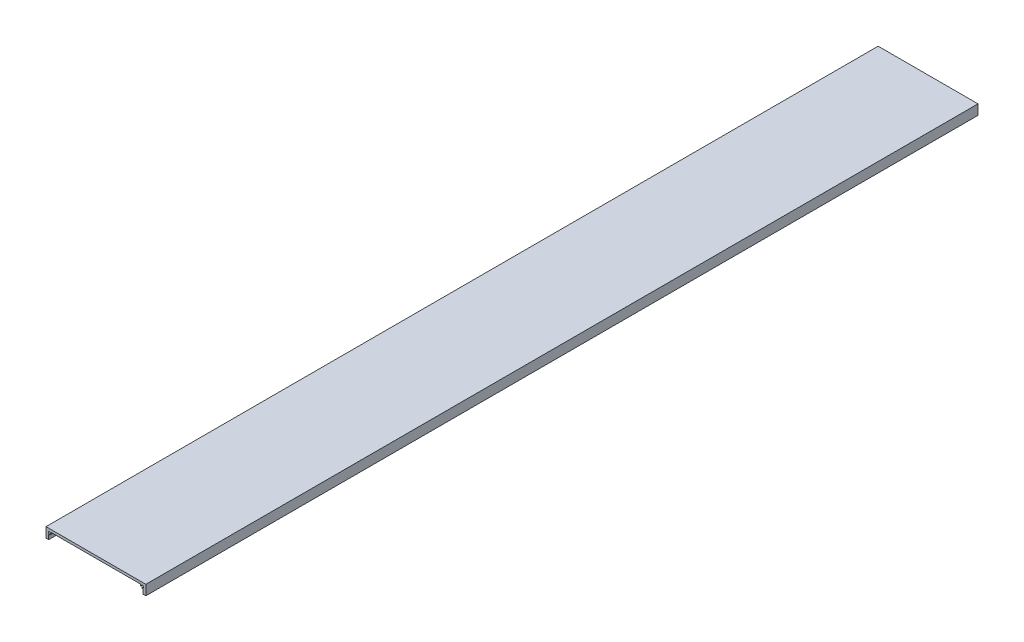
SolidWorks part; units mm, degrees
material "GY-D-120J型材"
ref_plane "前视基准面" through (0, 0, 0) normal (0, 0, 1) x (1, 0, 0)
ref_plane "上视基准面" through (0, 0, 0) normal (0, 1, 0) x (1, 0, 0)
ref_plane "右视基准面" through (0, 0, 0) normal (1, 0, 0) x (0, 0, -1)
sketch "草图1" plane through (0, 0, 0) normal (0, 0, 1) x (1, 0, 0)
  line L0 (0, 0) -> (0, 12) construction
  line L1 (60, 12) -> (-60, 12)
  line L2 (-60, 12) -> (-60, 0)
  line L3 (-60, 0) -> (-56.8, 0)
  line L4 (-56.8, 0) -> (-56.8, 5.5)
  line L5 (-56.8, 5.5) -> (-53.7, 5.5)
  line L6 (-53.7, 5.5) -> (-53.7, 9)
  line L7 (-53.7, 9) -> (53.7, 9)
  line L8 (53.7, 5.5) -> (53.7, 9)
  line L9 (56.8, 5.5) -> (53.7, 5.5)
  line L10 (56.8, 0) -> (56.8, 5.5)
  line L11 (60, 0) -> (56.8, 0)
  line L12 (60, 12) -> (60, 0)
  circle A0 centre (-56, 7.7) radius 1.25
  circle A1 centre (56, 7.7) radius 1.25
  point P11 (0, 9)
  dimension "D6" = 4
  dimension "D1" = 12
  dimension "D2" = 107.4
  dimension "D3" = 120
  dimension "D4" = 113.6
  dimension "D5" = 5.5
  dimension "D7" = 4.3
  dimension "D8" = 3
extrude "凸台-拉伸1" add sketch "草图1" along normal mid plane 1000
sketch "草图2" plane through (0, 0, 0) normal (0, 0, 1) x (1, 0, 0)
  line L0 (-53.7, 9) -> (53.7, 9) construction
  line L1 (-53.7, 5.5) -> (-55.4, 5.5)
  line L2 (-53.7, 5.5) -> (-53.7, 7.4)
  line L3 (-53.7, 7.4) -> (-55.4, 7.4)
  line L4 (-55.4, 5.5) -> (-55.4, 7.4)
  line L5 (-56.8, 0) -> (-56.8, 5.5) construction
  line L6 (0, 0) -> (0, 12) construction
  line L7 (60, 12) -> (-60, 12) construction
  line L8 (55.4, 5.5) -> (55.4, 7.4)
  line L9 (53.7, 7.4) -> (55.4, 7.4)
  line L10 (53.7, 5.5) -> (53.7, 7.4)
  line L11 (53.7, 5.5) -> (55.4, 5.5)
  dimension "D1" = 1.6
  dimension "D2" = 1.4
extrude "切除-拉伸1" cut sketch "草图2" along normal through all both and the other way through all
hole_wizard "M3 螺纹孔1" positions "草图8" profile "草图7" tap size "M3" standard "GB"
sketch "草图8" plane through (0, 0, 500) normal (0, 0, 1) x (1, 0, 0)
  point P0 (-56, 7.7)
  point P3 (56, 7.7)
sketch "草图7" plane through (-56, 7.7, 500) normal (1, 0, 0) x (0, -1, 0)
  line L0 (0, 0) -> (0, 20.7811)
  line L1 (0, 20.7811) -> (1.3, 20)
  line L2 (1.3, 20) -> (1.3, 0)
  line L5 (1.3, 0) -> (0, 0)
  line L10 (0, 20.7811) -> (-1.3, 20) construction
  line L11 (0, -6.35) -> (0, 107.95) construction
  dimension "螺纹孔钻头直径" = 2.6
  dimension "螺纹孔钻头深度" = 20
  dimension "导头角度" = 118
cosmetic thread "孔螺蚊线5" parameters "D1"=12, "D2"=3
cosmetic thread "孔螺蚊线6" parameters "D1"=12, "D2"=3
mirror "镜向1" about plane through (0, 0, 0) normal (0, 0, 1) of "M3 螺纹孔1"
